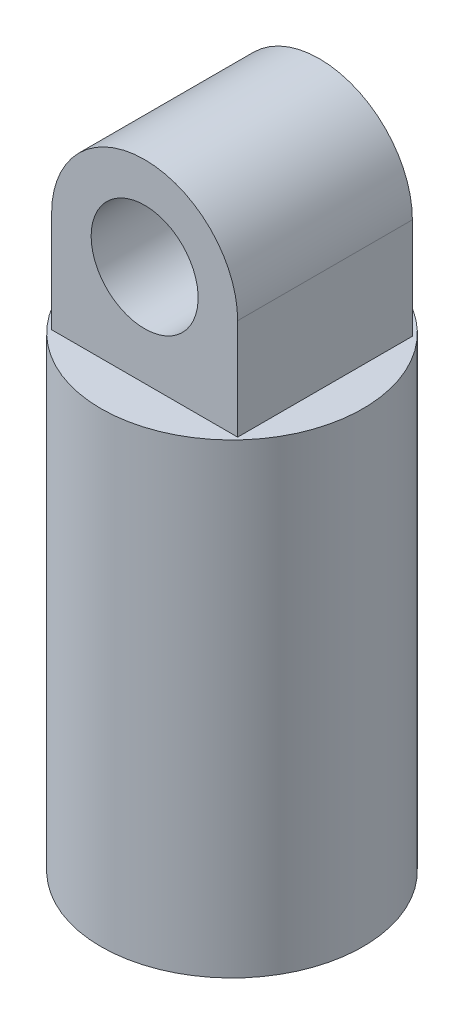
from build123d import *

# Parameters (mm, degrees)
BOSS_EXTRUDE1_DEPTH = 6
SKETCH3_R           = 9
BOSS_EXTRUDE2_DEPTH = 32
SKETCH5_R           = 3.674588618
CUT_EXTRUDE1_DEPTH  = 12


with BuildPart() as part:
    # Sketch2 → Boss-Extrude1 (new, symmetric)
    with BuildSketch(Plane(origin=(0, 0, 10.607757446), x_dir=(-1, 0, 0), z_dir=(0, 0, -1))):
        with BuildLine():
            Line((20.800074125, -16.288280471), (20.800074125, -23.215326818))
            Line((20.800074125, -23.215326818), (33.57764138, -23.215326818))
            Line((33.57764138, -23.215326818), (33.57764138, -16.288280471))
            ThreePointArc((33.57764138, -16.288280471), (27.188857752, -9.899496844), (20.800074125, -16.288280471))
        make_face()
    extrude(amount=BOSS_EXTRUDE1_DEPTH, both=True)

    # Sketch3 → Boss-Extrude2 (add)
    with BuildSketch(Plane.XZ.offset(23.215326818)):
        with Locations(Location((-27.188857752, 10.607757446, 0), (0, 0, 270))):
            Circle(SKETCH3_R)
    extrude(amount=BOSS_EXTRUDE2_DEPTH)

    # Sketch5 → Cut-Extrude1 (cut)
    with BuildSketch(Plane(origin=(0, 0, 4.607757446), x_dir=(-1, 0, 0), z_dir=(0, 0, -1))):
        with Locations((27.188857752, -16.288280471)):
            Circle(SKETCH5_R)
    extrude(amount=-CUT_EXTRUDE1_DEPTH, mode=Mode.SUBTRACT)


solid = part.part
